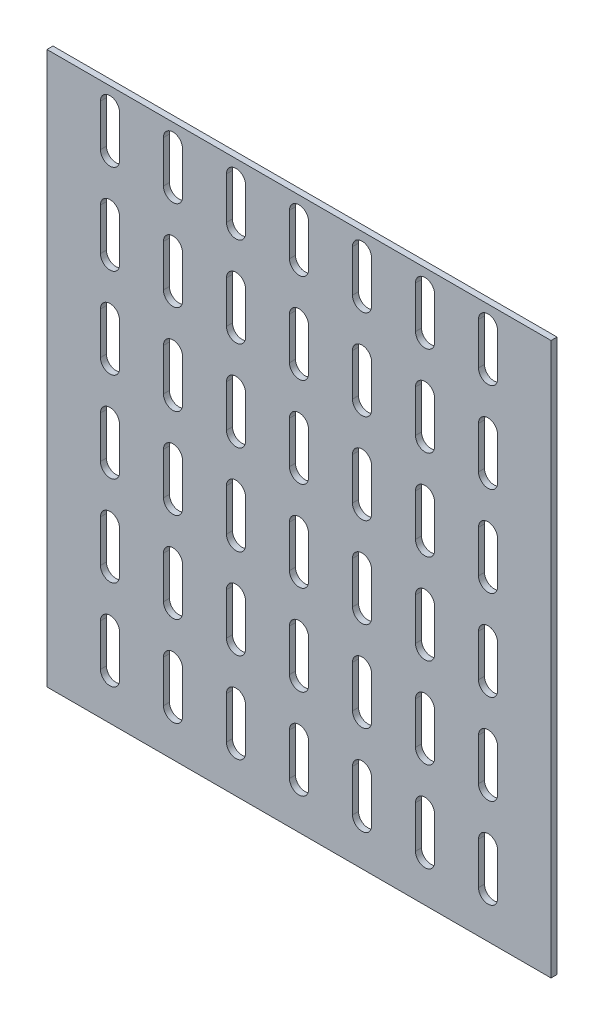
SolidWorks part; units mm, degrees
ref_plane "Front Plane" through (0, 0, 0) normal (0, 0, 1) x (1, 0, 0)
ref_plane "Top Plane" through (0, 0, 0) normal (0, 1, 0) x (1, 0, 0)
ref_plane "Right Plane" through (0, 0, 0) normal (1, 0, 0) x (0, 0, -1)
other "Configuration Table"
sketch "Sketch1" plane through (0, 0, 0) normal (0, 0, 1) x (1, 0, 0)
  line L0 (-51.062, 48.9899) -> (788.938, 48.9899)
  line L1 (788.938, 48.9899) -> (788.938, -871.0101)
  line L2 (788.938, -871.0101) -> (-51.062, -871.0101)
  line L3 (-51.062, -871.0101) -> (-51.062, 48.9899)
  dimension "D1" = 840
  dimension "D2" = 920
extrude "Boss-Extrude1" add sketch "Sketch1" along normal blind 10
sketch "Sketch2" plane through (0, 0, 10) normal (0, 0, 1) x (1, 0, 0)
  line L0 (53.938, -731.0101) -> (53.938, -801.0101) construction
  line L3 (69.8183, -731.0101) -> (69.8183, -801.0101)
  line L5 (38.0577, -731.0101) -> (38.0577, -801.0101)
  line L6 (158.938, -731.0101) -> (158.938, -801.0101) construction
  line L7 (174.8183, -731.0101) -> (174.8183, -801.0101)
  line L8 (158.938, 18.9899) -> (158.938, -51.0101) construction
  line L9 (69.8183, 18.9899) -> (69.8183, -51.0101)
  line L10 (38.0577, 18.9899) -> (38.0577, -51.0101)
  line L11 (174.8183, 18.9899) -> (174.8183, -51.0101)
  line L12 (143.0577, 18.9899) -> (143.0577, -51.0101)
  line L13 (263.938, 18.9899) -> (263.938, -51.0101) construction
  line L14 (279.8183, 18.9899) -> (279.8183, -51.0101)
  line L15 (248.0577, 18.9899) -> (248.0577, -51.0101)
  line L16 (368.938, 18.9899) -> (368.938, -51.0101) construction
  line L17 (384.8183, 18.9899) -> (384.8183, -51.0101)
  line L18 (353.0577, 18.9899) -> (353.0577, -51.0101)
  line L19 (473.938, 18.9899) -> (473.938, -51.0101) construction
  line L20 (489.8183, 18.9899) -> (489.8183, -51.0101)
  line L21 (458.0577, 18.9899) -> (458.0577, -51.0101)
  line L22 (578.938, 18.9899) -> (578.938, -51.0101) construction
  line L23 (594.8183, 18.9899) -> (594.8183, -51.0101)
  line L24 (563.0577, 18.9899) -> (563.0577, -51.0101)
  line L25 (683.938, 18.9899) -> (683.938, -51.0101) construction
  line L26 (699.8183, 18.9899) -> (699.8183, -51.0101)
  line L27 (668.0577, 18.9899) -> (668.0577, -51.0101)
  line L28 (53.938, -131.0101) -> (53.938, -201.0101) construction
  line L29 (69.8183, -131.0101) -> (69.8183, -201.0101)
  line L30 (38.0577, -131.0101) -> (38.0577, -201.0101)
  line L31 (158.938, -131.0101) -> (158.938, -201.0101) construction
  line L32 (174.8183, -131.0101) -> (174.8183, -201.0101)
  line L33 (143.0577, -131.0101) -> (143.0577, -201.0101)
  line L34 (263.938, -131.0101) -> (263.938, -201.0101) construction
  line L35 (279.8183, -131.0101) -> (279.8183, -201.0101)
  line L36 (248.0577, -131.0101) -> (248.0577, -201.0101)
  line L37 (368.938, -131.0101) -> (368.938, -201.0101) construction
  line L38 (384.8183, -131.0101) -> (384.8183, -201.0101)
  line L39 (353.0577, -131.0101) -> (353.0577, -201.0101)
  line L40 (473.938, -131.0101) -> (473.938, -201.0101) construction
  line L41 (489.8183, -131.0101) -> (489.8183, -201.0101)
  line L42 (458.0577, -131.0101) -> (458.0577, -201.0101)
  line L43 (578.938, -131.0101) -> (578.938, -201.0101) construction
  line L44 (594.8183, -131.0101) -> (594.8183, -201.0101)
  line L45 (563.0577, -131.0101) -> (563.0577, -201.0101)
  line L46 (683.938, -131.0101) -> (683.938, -201.0101) construction
  line L47 (699.8183, -131.0101) -> (699.8183, -201.0101)
  line L48 (668.0577, -131.0101) -> (668.0577, -201.0101)
  line L49 (53.938, -281.0101) -> (53.938, -351.0101) construction
  line L50 (69.8183, -281.0101) -> (69.8183, -351.0101)
  line L51 (38.0577, -281.0101) -> (38.0577, -351.0101)
  line L52 (158.938, -281.0101) -> (158.938, -351.0101) construction
  line L53 (174.8183, -281.0101) -> (174.8183, -351.0101)
  line L54 (143.0577, -281.0101) -> (143.0577, -351.0101)
  line L55 (263.938, -281.0101) -> (263.938, -351.0101) construction
  line L56 (279.8183, -281.0101) -> (279.8183, -351.0101)
  line L57 (248.0577, -281.0101) -> (248.0577, -351.0101)
  line L58 (368.938, -281.0101) -> (368.938, -351.0101) construction
  line L59 (384.8183, -281.0101) -> (384.8183, -351.0101)
  line L60 (353.0577, -281.0101) -> (353.0577, -351.0101)
  line L61 (473.938, -281.0101) -> (473.938, -351.0101) construction
  line L62 (489.8183, -281.0101) -> (489.8183, -351.0101)
  line L63 (458.0577, -281.0101) -> (458.0577, -351.0101)
  line L64 (578.938, -281.0101) -> (578.938, -351.0101) construction
  line L65 (594.8183, -281.0101) -> (594.8183, -351.0101)
  line L66 (563.0577, -281.0101) -> (563.0577, -351.0101)
  line L67 (683.938, -281.0101) -> (683.938, -351.0101) construction
  line L68 (699.8183, -281.0101) -> (699.8183, -351.0101)
  line L69 (668.0577, -281.0101) -> (668.0577, -351.0101)
  line L70 (53.938, -431.0101) -> (53.938, -501.0101) construction
  line L71 (69.8183, -431.0101) -> (69.8183, -501.0101)
  line L72 (38.0577, -431.0101) -> (38.0577, -501.0101)
  line L73 (158.938, -431.0101) -> (158.938, -501.0101) construction
  line L74 (174.8183, -431.0101) -> (174.8183, -501.0101)
  line L75 (143.0577, -431.0101) -> (143.0577, -501.0101)
  line L76 (263.938, -431.0101) -> (263.938, -501.0101) construction
  line L77 (279.8183, -431.0101) -> (279.8183, -501.0101)
  line L78 (248.0577, -431.0101) -> (248.0577, -501.0101)
  line L79 (368.938, -431.0101) -> (368.938, -501.0101) construction
  line L80 (384.8183, -431.0101) -> (384.8183, -501.0101)
  line L81 (353.0577, -431.0101) -> (353.0577, -501.0101)
  line L82 (473.938, -431.0101) -> (473.938, -501.0101) construction
  line L83 (489.8183, -431.0101) -> (489.8183, -501.0101)
  line L84 (458.0577, -431.0101) -> (458.0577, -501.0101)
  line L85 (578.938, -431.0101) -> (578.938, -501.0101) construction
  line L86 (594.8183, -431.0101) -> (594.8183, -501.0101)
  line L87 (563.0577, -431.0101) -> (563.0577, -501.0101)
  line L88 (683.938, -431.0101) -> (683.938, -501.0101) construction
  line L89 (699.8183, -431.0101) -> (699.8183, -501.0101)
  line L90 (668.0577, -431.0101) -> (668.0577, -501.0101)
  line L91 (53.938, -581.0101) -> (53.938, -651.0101) construction
  line L92 (69.8183, -581.0101) -> (69.8183, -651.0101)
  line L93 (38.0577, -581.0101) -> (38.0577, -651.0101)
  line L94 (158.938, -581.0101) -> (158.938, -651.0101) construction
  line L95 (174.8183, -581.0101) -> (174.8183, -651.0101)
  line L96 (143.0577, -581.0101) -> (143.0577, -651.0101)
  line L97 (263.938, -581.0101) -> (263.938, -651.0101) construction
  line L98 (279.8183, -581.0101) -> (279.8183, -651.0101)
  line L99 (248.0577, -581.0101) -> (248.0577, -651.0101)
  line L100 (368.938, -581.0101) -> (368.938, -651.0101) construction
  line L101 (384.8183, -581.0101) -> (384.8183, -651.0101)
  line L102 (353.0577, -581.0101) -> (353.0577, -651.0101)
  line L103 (473.938, -581.0101) -> (473.938, -651.0101) construction
  line L104 (489.8183, -581.0101) -> (489.8183, -651.0101)
  line L105 (458.0577, -581.0101) -> (458.0577, -651.0101)
  line L106 (578.938, -581.0101) -> (578.938, -651.0101) construction
  line L107 (594.8183, -581.0101) -> (594.8183, -651.0101)
  line L108 (563.0577, -581.0101) -> (563.0577, -651.0101)
  line L109 (683.938, -581.0101) -> (683.938, -651.0101) construction
  line L110 (699.8183, -581.0101) -> (699.8183, -651.0101)
  line L111 (668.0577, -581.0101) -> (668.0577, -651.0101)
  line L112 (143.0577, -731.0101) -> (143.0577, -801.0101)
  line L113 (263.938, -731.0101) -> (263.938, -801.0101) construction
  line L114 (279.8183, -731.0101) -> (279.8183, -801.0101)
  line L115 (248.0577, -731.0101) -> (248.0577, -801.0101)
  line L116 (368.938, -731.0101) -> (368.938, -801.0101) construction
  line L117 (384.8183, -731.0101) -> (384.8183, -801.0101)
  line L118 (353.0577, -731.0101) -> (353.0577, -801.0101)
  line L119 (473.938, -731.0101) -> (473.938, -801.0101) construction
  line L120 (489.8183, -731.0101) -> (489.8183, -801.0101)
  line L121 (458.0577, -731.0101) -> (458.0577, -801.0101)
  line L122 (578.938, -731.0101) -> (578.938, -801.0101) construction
  line L123 (594.8183, -731.0101) -> (594.8183, -801.0101)
  line L124 (563.0577, -731.0101) -> (563.0577, -801.0101)
  line L125 (683.938, -731.0101) -> (683.938, -801.0101) construction
  line L126 (699.8183, -731.0101) -> (699.8183, -801.0101)
  line L127 (668.0577, -731.0101) -> (668.0577, -801.0101)
  arc A0 (69.8183, 18.9899) -> (38.0577, 18.9899) centre (53.938, 18.9899) ccw
  arc A1 (38.0577, -51.0101) -> (69.8183, -51.0101) centre (53.938, -51.0101) ccw
  arc A2 (174.8183, 18.9899) -> (143.0577, 18.9899) centre (158.938, 18.9899) ccw
  arc A3 (143.0577, -51.0101) -> (174.8183, -51.0101) centre (158.938, -51.0101) ccw
  arc A4 (279.8183, 18.9899) -> (248.0577, 18.9899) centre (263.938, 18.9899) ccw
  arc A5 (248.0577, -51.0101) -> (279.8183, -51.0101) centre (263.938, -51.0101) ccw
  arc A6 (384.8183, 18.9899) -> (353.0577, 18.9899) centre (368.938, 18.9899) ccw
  arc A7 (353.0577, -51.0101) -> (384.8183, -51.0101) centre (368.938, -51.0101) ccw
  arc A8 (489.8183, 18.9899) -> (458.0577, 18.9899) centre (473.938, 18.9899) ccw
  arc A9 (458.0577, -51.0101) -> (489.8183, -51.0101) centre (473.938, -51.0101) ccw
  arc A10 (594.8183, 18.9899) -> (563.0577, 18.9899) centre (578.938, 18.9899) ccw
  arc A11 (563.0577, -51.0101) -> (594.8183, -51.0101) centre (578.938, -51.0101) ccw
  arc A12 (699.8183, 18.9899) -> (668.0577, 18.9899) centre (683.938, 18.9899) ccw
  arc A13 (668.0577, -51.0101) -> (699.8183, -51.0101) centre (683.938, -51.0101) ccw
  arc A14 (69.8183, -131.0101) -> (38.0577, -131.0101) centre (53.938, -131.0101) ccw
  arc A15 (38.0577, -201.0101) -> (69.8183, -201.0101) centre (53.938, -201.0101) ccw
  arc A16 (174.8183, -131.0101) -> (143.0577, -131.0101) centre (158.938, -131.0101) ccw
  arc A17 (143.0577, -201.0101) -> (174.8183, -201.0101) centre (158.938, -201.0101) ccw
  arc A18 (279.8183, -131.0101) -> (248.0577, -131.0101) centre (263.938, -131.0101) ccw
  arc A19 (248.0577, -201.0101) -> (279.8183, -201.0101) centre (263.938, -201.0101) ccw
  arc A20 (384.8183, -131.0101) -> (353.0577, -131.0101) centre (368.938, -131.0101) ccw
  arc A21 (353.0577, -201.0101) -> (384.8183, -201.0101) centre (368.938, -201.0101) ccw
  arc A22 (489.8183, -131.0101) -> (458.0577, -131.0101) centre (473.938, -131.0101) ccw
  arc A23 (458.0577, -201.0101) -> (489.8183, -201.0101) centre (473.938, -201.0101) ccw
  arc A24 (594.8183, -131.0101) -> (563.0577, -131.0101) centre (578.938, -131.0101) ccw
  arc A25 (563.0577, -201.0101) -> (594.8183, -201.0101) centre (578.938, -201.0101) ccw
  arc A26 (699.8183, -131.0101) -> (668.0577, -131.0101) centre (683.938, -131.0101) ccw
  arc A27 (668.0577, -201.0101) -> (699.8183, -201.0101) centre (683.938, -201.0101) ccw
  arc A28 (69.8183, -281.0101) -> (38.0577, -281.0101) centre (53.938, -281.0101) ccw
  arc A29 (38.0577, -351.0101) -> (69.8183, -351.0101) centre (53.938, -351.0101) ccw
  arc A30 (174.8183, -281.0101) -> (143.0577, -281.0101) centre (158.938, -281.0101) ccw
  arc A31 (143.0577, -351.0101) -> (174.8183, -351.0101) centre (158.938, -351.0101) ccw
  arc A32 (279.8183, -281.0101) -> (248.0577, -281.0101) centre (263.938, -281.0101) ccw
  arc A33 (248.0577, -351.0101) -> (279.8183, -351.0101) centre (263.938, -351.0101) ccw
  arc A34 (384.8183, -281.0101) -> (353.0577, -281.0101) centre (368.938, -281.0101) ccw
  arc A35 (353.0577, -351.0101) -> (384.8183, -351.0101) centre (368.938, -351.0101) ccw
  arc A36 (489.8183, -281.0101) -> (458.0577, -281.0101) centre (473.938, -281.0101) ccw
  arc A37 (458.0577, -351.0101) -> (489.8183, -351.0101) centre (473.938, -351.0101) ccw
  arc A38 (594.8183, -281.0101) -> (563.0577, -281.0101) centre (578.938, -281.0101) ccw
  arc A39 (563.0577, -351.0101) -> (594.8183, -351.0101) centre (578.938, -351.0101) ccw
  arc A40 (699.8183, -281.0101) -> (668.0577, -281.0101) centre (683.938, -281.0101) ccw
  arc A41 (668.0577, -351.0101) -> (699.8183, -351.0101) centre (683.938, -351.0101) ccw
  arc A42 (69.8183, -431.0101) -> (38.0577, -431.0101) centre (53.938, -431.0101) ccw
  arc A43 (38.0577, -501.0101) -> (69.8183, -501.0101) centre (53.938, -501.0101) ccw
  arc A44 (174.8183, -431.0101) -> (143.0577, -431.0101) centre (158.938, -431.0101) ccw
  arc A45 (143.0577, -501.0101) -> (174.8183, -501.0101) centre (158.938, -501.0101) ccw
  arc A46 (279.8183, -431.0101) -> (248.0577, -431.0101) centre (263.938, -431.0101) ccw
  arc A47 (248.0577, -501.0101) -> (279.8183, -501.0101) centre (263.938, -501.0101) ccw
  arc A48 (384.8183, -431.0101) -> (353.0577, -431.0101) centre (368.938, -431.0101) ccw
  arc A49 (353.0577, -501.0101) -> (384.8183, -501.0101) centre (368.938, -501.0101) ccw
  arc A50 (489.8183, -431.0101) -> (458.0577, -431.0101) centre (473.938, -431.0101) ccw
  arc A51 (458.0577, -501.0101) -> (489.8183, -501.0101) centre (473.938, -501.0101) ccw
  arc A52 (594.8183, -431.0101) -> (563.0577, -431.0101) centre (578.938, -431.0101) ccw
  arc A53 (563.0577, -501.0101) -> (594.8183, -501.0101) centre (578.938, -501.0101) ccw
  arc A54 (699.8183, -431.0101) -> (668.0577, -431.0101) centre (683.938, -431.0101) ccw
  arc A55 (668.0577, -501.0101) -> (699.8183, -501.0101) centre (683.938, -501.0101) ccw
  arc A56 (69.8183, -581.0101) -> (38.0577, -581.0101) centre (53.938, -581.0101) ccw
  arc A57 (38.0577, -651.0101) -> (69.8183, -651.0101) centre (53.938, -651.0101) ccw
  arc A58 (174.8183, -581.0101) -> (143.0577, -581.0101) centre (158.938, -581.0101) ccw
  arc A59 (143.0577, -651.0101) -> (174.8183, -651.0101) centre (158.938, -651.0101) ccw
  arc A60 (279.8183, -581.0101) -> (248.0577, -581.0101) centre (263.938, -581.0101) ccw
  arc A61 (248.0577, -651.0101) -> (279.8183, -651.0101) centre (263.938, -651.0101) ccw
  arc A62 (384.8183, -581.0101) -> (353.0577, -581.0101) centre (368.938, -581.0101) ccw
  arc A63 (353.0577, -651.0101) -> (384.8183, -651.0101) centre (368.938, -651.0101) ccw
  arc A64 (489.8183, -581.0101) -> (458.0577, -581.0101) centre (473.938, -581.0101) ccw
  arc A65 (458.0577, -651.0101) -> (489.8183, -651.0101) centre (473.938, -651.0101) ccw
  arc A66 (594.8183, -581.0101) -> (563.0577, -581.0101) centre (578.938, -581.0101) ccw
  arc A67 (563.0577, -651.0101) -> (594.8183, -651.0101) centre (578.938, -651.0101) ccw
  arc A68 (699.8183, -581.0101) -> (668.0577, -581.0101) centre (683.938, -581.0101) ccw
  arc A69 (668.0577, -651.0101) -> (699.8183, -651.0101) centre (683.938, -651.0101) ccw
  arc A70 (69.8183, -731.0101) -> (38.0577, -731.0101) centre (53.938, -731.0101) ccw
  arc A71 (38.0577, -801.0101) -> (69.8183, -801.0101) centre (53.938, -801.0101) ccw
  arc A72 (174.8183, -731.0101) -> (143.0577, -731.0101) centre (158.938, -731.0101) ccw
  arc A73 (143.0577, -801.0101) -> (174.8183, -801.0101) centre (158.938, -801.0101) ccw
  arc A74 (279.8183, -731.0101) -> (248.0577, -731.0101) centre (263.938, -731.0101) ccw
  arc A75 (248.0577, -801.0101) -> (279.8183, -801.0101) centre (263.938, -801.0101) ccw
  arc A76 (384.8183, -731.0101) -> (353.0577, -731.0101) centre (368.938, -731.0101) ccw
  arc A77 (353.0577, -801.0101) -> (384.8183, -801.0101) centre (368.938, -801.0101) ccw
  arc A78 (489.8183, -731.0101) -> (458.0577, -731.0101) centre (473.938, -731.0101) ccw
  arc A79 (458.0577, -801.0101) -> (489.8183, -801.0101) centre (473.938, -801.0101) ccw
  arc A80 (594.8183, -731.0101) -> (563.0577, -731.0101) centre (578.938, -731.0101) ccw
  arc A81 (563.0577, -801.0101) -> (594.8183, -801.0101) centre (578.938, -801.0101) ccw
  arc A82 (699.8183, -731.0101) -> (668.0577, -731.0101) centre (683.938, -731.0101) ccw
  arc A83 (668.0577, -801.0101) -> (699.8183, -801.0101) centre (683.938, -801.0101) ccw
  point P4 (53.938, -766.0101)
  point P11 (158.938, -766.0101)
  point P18 (53.938, -16.0101)
  point P25 (158.938, -16.0101)
  point P32 (263.938, -16.0101)
  point P39 (368.938, -16.0101)
  point P46 (473.938, -16.0101)
  point P53 (578.938, -16.0101)
  point P60 (683.938, -16.0101)
  point P67 (53.938, -166.0101)
  point P74 (158.938, -166.0101)
  point P81 (263.938, -166.0101)
  point P88 (368.938, -166.0101)
  point P95 (473.938, -166.0101)
  point P102 (578.938, -166.0101)
  point P109 (683.938, -166.0101)
  point P116 (53.938, -316.0101)
  point P123 (158.938, -316.0101)
  point P130 (263.938, -316.0101)
  point P137 (368.938, -316.0101)
  point P144 (473.938, -316.0101)
  point P151 (578.938, -316.0101)
  point P158 (683.938, -316.0101)
  point P165 (53.938, -466.0101)
  point P172 (158.938, -466.0101)
  point P179 (263.938, -466.0101)
  point P186 (368.938, -466.0101)
  point P193 (473.938, -466.0101)
  point P200 (578.938, -466.0101)
  point P207 (683.938, -466.0101)
  point P214 (53.938, -616.0101)
  point P221 (158.938, -616.0101)
  point P228 (263.938, -616.0101)
  point P235 (368.938, -616.0101)
  point P242 (473.938, -616.0101)
  point P249 (578.938, -616.0101)
  point P256 (683.938, -616.0101)
  point P263 (263.938, -766.0101)
  point P270 (368.938, -766.0101)
  point P277 (473.938, -766.0101)
  point P284 (578.938, -766.0101)
  point P291 (683.938, -766.0101)
  dimension "D1" = 2
  dimension "D5" = 5
extrude "Cut-Extrude1" cut sketch "Sketch2" against normal blind 10 contours L10 A1 L9 A0 | L11 A3 L12 A2 | L14 A5 L15 A4 | L17 A7 L18 A6 | L20 A9 L21 A8 | L23 A11 L24 A10 | L26 A13 L27 A12 | L47 A27 L48 A26 | L44 A25 L45 A24 | L41 A23 L42 A22 | L38 A21 L39 A20 | L35 A19 L36 A18 | L32 A17 L33 A16 | L29 A15 L30 A14 | L50 A29 L51 A28 | L53 A31 L54 A30 | L56 A33 L57 A32 | L59 A35 L60 A34 | L62 A37 L63 A36 | L65 A39 L66 A38 | L68 A41 L69 A40 | L71 A43 L72 A42 | L74 A45 L75 A44 | L77 A47 L78 A46 | L80 A49 L81 A48 | L83 A51 L84 A50 | L89 A55 L90 A54 | L86 A53 L87 A52 | L107 A67 L108 A66 | L110 A69 L111 A68 | L104 A65 L105 A64 | L101 A63 L102 A62 | L95 A59 L96 A58 | L98 A61 L99 A60 | L92 A57 L93 A56 | L3 A71 L5 A70 | L7 A73 L112 A72 | L114 A75 L115 A74 | L117 A77 L118 A76 | L120 A79 L121 A78 | L123 A81 L124 A80 | L126 A83 L127 A82
